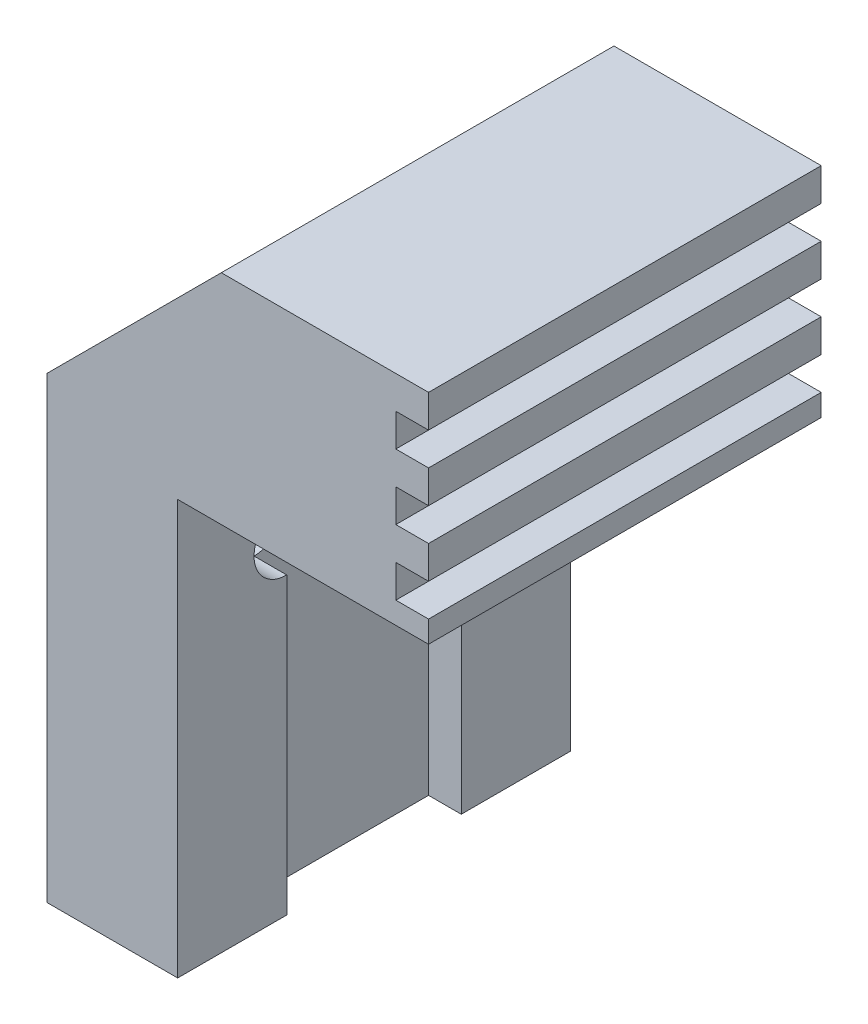
from build123d import *

# Parameters (mm, degrees)
EXTRUDE_1_DEPTH     = 9
SKETCH_2_W          = 8
SKETCH_2_H          = 15
CUT_EXTRUDE_1_DEPTH = 1.5
CUT_EXTRUDE_2_REACH = 34.469
SKETCH_3_R          = 1.5
SKETCH_4_W          = 18
SKETCH_4_H          = 1.5
CUT_EXTRUDE_3_DEPTH = 1.5
CHAMFER_1_SIZE      = 8


with BuildPart() as part:
    # 草图1 → 凸台-拉伸1 (new, symmetric)
    with BuildSketch(Plane.XY):
        Polygon((0, 0), (0, 29), (17.5, 29), (17.5, 19), (6, 19), (6, 0), align=None)
    extrude(amount=EXTRUDE_1_DEPTH, both=True)

    # 草图2 → 切除-拉伸1 (cut)
    with BuildSketch(Plane(origin=(6, 0, 0), x_dir=(0, 0, -1), z_dir=(1, 0, 0))):
        with Locations((0, 7.5)):
            Rectangle(SKETCH_2_W, SKETCH_2_H)
    extrude(amount=-CUT_EXTRUDE_1_DEPTH, mode=Mode.SUBTRACT)

    # 草图3 → 切除-拉伸2 (cut, up to next)
    with BuildSketch(Plane(origin=(6, 0, 0), x_dir=(0, 0, -1), z_dir=(1, 0, 0)), mode=Mode.PRIVATE) as cut_extrude_2_sk1:
        with Locations(Location((4, 15, 0), (0, 0, 180))):
            Circle(SKETCH_3_R)
    cut_extrude_2_tool1 = extrude(cut_extrude_2_sk1.sketch, amount=-CUT_EXTRUDE_2_REACH, mode=Mode.PRIVATE) & part.part
    # 草图3 → 切除-拉伸2 (cut, up to next)
    with BuildSketch(Plane(origin=(6, 0, 0), x_dir=(0, 0, -1), z_dir=(1, 0, 0)), mode=Mode.PRIVATE) as cut_extrude_2_sk2:
        with Locations((-4, 15)):
            Circle(SKETCH_3_R)
    cut_extrude_2_tool2 = extrude(cut_extrude_2_sk2.sketch, amount=-CUT_EXTRUDE_2_REACH, mode=Mode.PRIVATE) & part.part
    add(cut_extrude_2_tool1.solids().sort_by_distance((6, 15, -4))[0], mode=Mode.SUBTRACT)
    add(cut_extrude_2_tool2.solids().sort_by_distance((6, 15, 4))[0], mode=Mode.SUBTRACT)

    # 草图4 → 切除-拉伸3 (cut)
    with BuildSketch(Plane(origin=(17.5, 0, 0), x_dir=(0, 0, -1), z_dir=(1, 0, 0))):
        with Locations((0, 26.75)):
            Rectangle(SKETCH_4_W, SKETCH_4_H)
        with Locations((0, 23.75)):
            Rectangle(SKETCH_4_W, SKETCH_4_H)
        with Locations((0, 20.75)):
            Rectangle(SKETCH_4_W, SKETCH_4_H)
    extrude(amount=-CUT_EXTRUDE_3_DEPTH, mode=Mode.SUBTRACT)

    # 倒角1
    chamfer_1_edges = [part.edges().sort_by_distance(p)[0] for p in [
        (0, 29, 0),
    ]]
    chamfer(chamfer_1_edges, length=CHAMFER_1_SIZE)


solid = part.part
